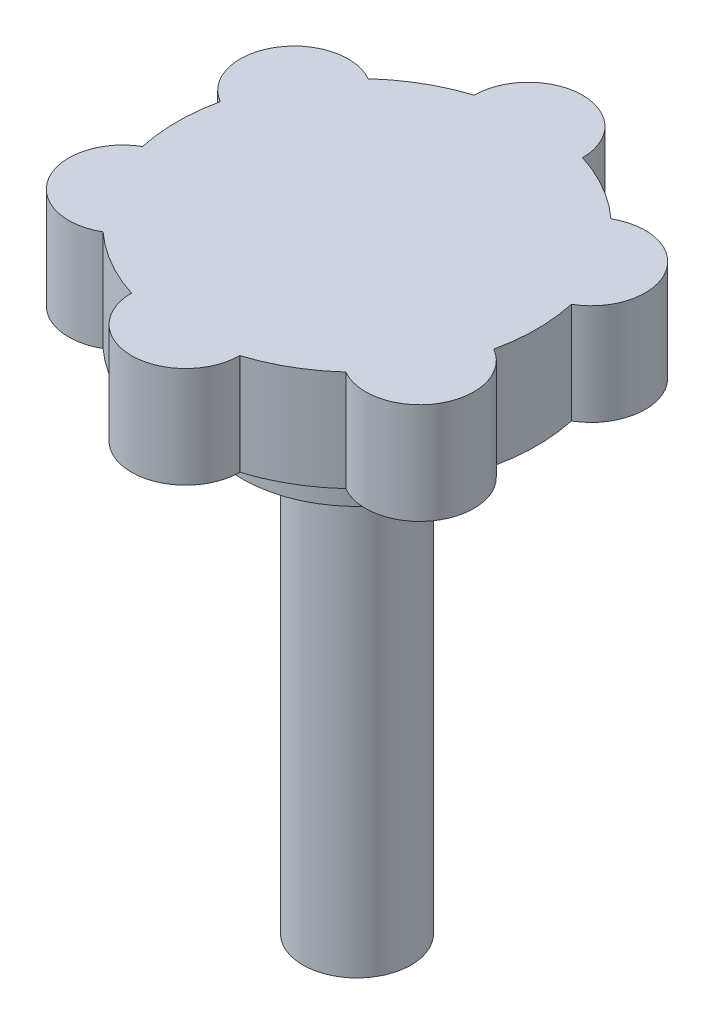
SolidWorks part; units mm, degrees
ref_plane "Front Plane" through (0, 0, 0) normal (0, 0, 1) x (1, 0, 0)
ref_plane "Top Plane" through (0, 0, 0) normal (0, 1, 0) x (1, 0, 0)
ref_plane "Right Plane" through (0, 0, 0) normal (1, 0, 0) x (0, 0, -1)
sketch "Sketch1" plane through (0, 0, 0) normal (0, 1, 0) x (1, 0, 0)
  line L21 (-6.7261, 7.3469) -> (-6.7267, 7.3472)
  line L22 (-3, 9.4991) -> (-3, 9.5)
  line L23 (6.7272, 7.3486) -> (6.7277, 7.3489)
  line L24 (-9.7242, -2.1519) -> (-9.7257, -2.1528)
  line L25 (-9.725, 2.1501) -> (-9.7267, 2.1511)
  line L26 (-2.998, -9.498) -> (-2.998, -9.5)
  line L27 (-6.7234, -7.3476) -> (-6.7257, -7.3489)
  line L28 (6.7276, -7.3465) -> (6.7287, -7.3472)
  line L29 (3.002, -9.4976) -> (3.002, -9.5)
  line L30 (9.7275, 2.1526) -> (9.7277, 2.1528)
  line L31 (9.7276, -2.1504) -> (9.7287, -2.1511)
  arc A2 (3, 9.5) -> (-3, 9.5) centre (0, 9.5) ccw
  arc A4 (9.7277, 2.1528) -> (6.7277, 7.3489) centre (8.2277, 4.7509) ccw
  arc A6 (6.7287, -7.3472) -> (9.7287, -2.1511) centre (8.2287, -4.7491) ccw
  arc A8 (-2.998, -9.5) -> (3.002, -9.5) centre (0.002, -9.5) ccw
  arc A10 (-9.7257, -2.1528) -> (-6.7257, -7.3489) centre (-8.2257, -4.7509) ccw
  arc A12 (-6.7267, 7.3472) -> (-9.7267, 2.1511) centre (-8.2267, 4.7491) ccw
  arc A13 (-9.725, 2.1501) -> (-9.7242, -2.1519) centre (0.0015, 0.0009) ccw
  arc A17 (-3, 9.4991) -> (-6.7261, 7.3469) centre (0.0015, 0.0009) ccw
  arc A18 (6.7272, 7.3486) -> (3, 9.5) centre (0.0015, 0.0009) ccw
  arc A22 (-6.7234, -7.3476) -> (-2.998, -9.498) centre (0.0015, 0.0009) ccw
  arc A25 (3.002, -9.4976) -> (6.7276, -7.3465) centre (0.0015, 0.0009) ccw
  arc A26 (9.7276, -2.1504) -> (9.7275, 2.1526) centre (0.0015, 0.0009) ccw
  point P53 (-4.1131, 2.3741)
  dimension "D2" = 3
extrude "Boss-Extrude1" add sketch "Sketch1" along normal blind 5.6
sketch "Sketch2" plane through (0, 0, 0) normal (0, -1, 0) x (1, 0, 0)
  circle A0 centre (0, 0) radius 6.35
  dimension "D1" = 12.7
extrude "Boss-Extrude2" add sketch "Sketch2" along normal blind 3.4
sketch "Sketch3" plane through (0, -3.4, 0) normal (0, -1, 0) x (1, 0, 0)
  circle A0 centre (0, 0) radius 3
  dimension "D1" = 6
extrude "Boss-Extrude3" add sketch "Sketch3" along normal blind 25
